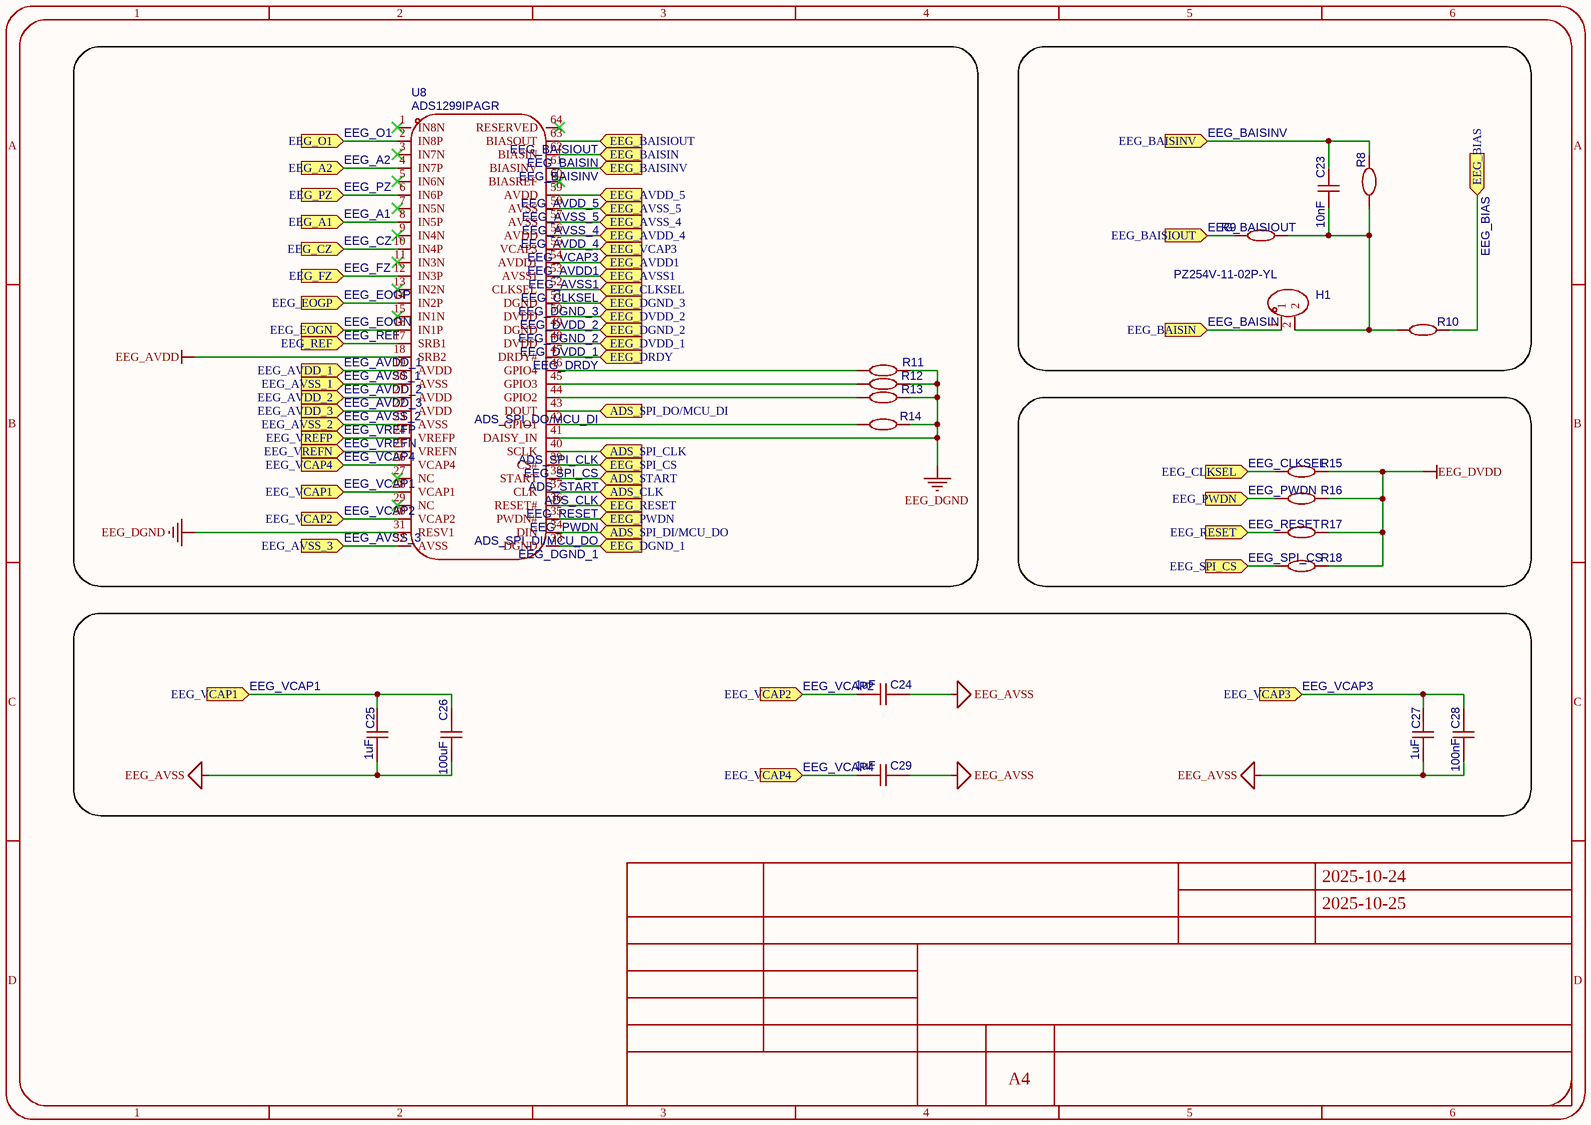
[diagram p0: MISC86293-4.schdoc]
# Altium project MISC86293-17.PrjPCB (part 2 of 3)

## Sheet MISC86293-4.schdoc
size 297 x 209 mm; @Create Time: 20:02:05; @Update Time: 00:34:01; @Board Name: MISC86293; Version: V1.0; @Project Name: MISC86293; @Page Count: 8; @Update Date: 2025-10-25; @Create Date: 2025-10-24; @Schematic Name: MISC86293; @Page No: 2

### Parts
C23  10nF  [C0402]
C24  1uF  [C0402]
C25  1uF  [C0402]
C26  100uF  [C1206]
C27  1uF  [C0402]
C28  100nF  [C0402]
C29  1uF  [C0402]
H1  PZ254V-11-02P-YL  [HDR-TH_2P-P2.54-V-M]
R8  (no value)  [R0402]
R9  (no value)  [R0402]
R10  (no value)  [R0402]
R11  (no value)  [R0402]
R12  (no value)  [R0402]
R13  (no value)  [R0402]
R14  (no value)  [R0402]
R15  (no value)  [R0402]
R16  (no value)  [R0402]
R17  (no value)  [R0402]
R18  (no value)  [R0402]
U8  ADS1299IPAGR  [TQFP-64_L10.0-W10.0-P0.50-LS12.0-TL]

### Ports
ADS_CLK (in), ADS_SPI_CLK (in), ADS_SPI_DI/MCU_DO (in), ADS_SPI_DO/MCU_DI (in), ADS_START (in), EEG_A1 (in), EEG_A2 (in), EEG_AVDD1 (in), EEG_AVDD_1 (in), EEG_AVDD_2 (in), EEG_AVDD_3 (in), EEG_AVDD_4 (in), EEG_AVDD_5 (in), EEG_AVSS1 (in), EEG_AVSS_1 (in), EEG_AVSS_2 (in), EEG_AVSS_3 (in), EEG_AVSS_4 (in), EEG_AVSS_5 (in), EEG_BAISIN (in), EEG_BAISINV (in), EEG_BAISIOUT (in), EEG_BIAS (in), EEG_CLKSEL (in), EEG_CZ (in), EEG_DGND_1 (in), EEG_DGND_2 (in), EEG_DGND_3 (in), EEG_DRDY (in), EEG_DVDD_1 (in), EEG_DVDD_2 (in), EEG_EOGN (in), EEG_EOGP (in), EEG_FZ (in), EEG_O1 (in), EEG_PWDN (in), EEG_PZ (in), EEG_REF (in), EEG_RESET (in), EEG_SPI_CS (in), EEG_VCAP1 (in), EEG_VCAP2 (in), EEG_VCAP3 (in), EEG_VCAP4 (in), EEG_VREFN (in), EEG_VREFP (in)

### Nets
EEG_AVDD1: U8.18(SRB2) U8.19(AVDD) U8.21(AVDD) U8.22(AVDD) U8.54(AVDD1) U8.56(AVDD) U8.59(AVDD) ; port EEG_AVDD_1, port EEG_AVDD_2, port EEG_AVDD_3, port EEG_AVDD_4, port EEG_AVDD_5, port EEG_AVDD1  [also labelled EEG_AVDD, EEG_AVDD_1, EEG_AVDD_2, EEG_AVDD_3, EEG_AVDD_4, EEG_AVDD_5]
EEG_AVSS1: C24.2 C25.1 C26.1 C27.1 C28.1 C29.2 U8.20(AVSS) U8.23(AVSS) U8.25(VREFN) U8.32(AVSS) U8.53(AVSS1) U8.57(AVSS) U8.58(AVSS) ; port EEG_AVSS_1, port EEG_AVSS_2, port EEG_AVSS_4, port EEG_AVSS_5, port EEG_AVSS1, port EEG_VREFN, port EEG_AVSS_3  [also labelled EEG_AVSS, EEG_AVSS_1, EEG_AVSS_2, EEG_AVSS_3, EEG_AVSS_4, EEG_AVSS_5, EEG_VREFN]
EEG_DGND_1: R11.2 R12.2 R13.2 R14.2 U8.31(RESV1) U8.33(DGND) U8.41(DAISY_IN) U8.49(DGND) U8.51(DGND) ; port EEG_DGND_1, port EEG_DGND_2, port EEG_DGND_3  [also labelled EEG_DGND, EEG_DGND_2, EEG_DGND_3]
EEG_DVDD_1: R15.2 R16.2 R17.2 R18.2 U8.48(DVDD) U8.50(DVDD) ; port EEG_DVDD_1, port EEG_DVDD_2  [also labelled EEG_DVDD, EEG_DVDD_2]
ADS_CLK: U8.37(CLK) ; port ADS_CLK
ADS_SPI_CLK: U8.40(SCLK) ; port ADS_SPI_CLK
ADS_SPI_DI/MCU_DO: U8.34(DIN) ; port ADS_SPI_DI/MCU_DO
ADS_SPI_DO/MCU_DI: U8.43(DOUT) ; port ADS_SPI_DO/MCU_DI
ADS_START: U8.38(START) ; port ADS_START
EEG_A1: U8.8(IN5P) ; port EEG_A1
EEG_A2: U8.4(IN7P) ; port EEG_A2
EEG_BAISIN: H1.1 U8.62(BIASIN) ; port EEG_BAISIN
EEG_BAISINV: C23.2 R8.1 U8.61(BIASINV) ; port EEG_BAISINV
EEG_BAISIOUT: R9.1 U8.63(BIASOUT) ; port EEG_BAISIOUT
EEG_BIAS: R10.2 ; port EEG_BIAS
EEG_CLKSEL: R15.1 U8.52(CLKSEL) ; port EEG_CLKSEL
EEG_CZ: U8.10(IN4P) ; port EEG_CZ
EEG_DRDY: U8.47(DRDY#) ; port EEG_DRDY
EEG_EOGN: U8.16(IN1P) ; port EEG_EOGN
EEG_EOGP: U8.14(IN2P) ; port EEG_EOGP
EEG_FZ: U8.12(IN3P) ; port EEG_FZ
EEG_O1: U8.2(IN8P) ; port EEG_O1
EEG_PWDN: R16.1 U8.35(PWDN#) ; port EEG_PWDN
EEG_PZ: U8.6(IN6P) ; port EEG_PZ
EEG_REF: U8.17(SRB1) ; port EEG_REF
EEG_RESET: R17.1 U8.36(RESET#) ; port EEG_RESET
EEG_SPI_CS: R18.1 U8.39(CS#) ; port EEG_SPI_CS
EEG_VCAP1: C25.2 C26.2 U8.28(VCAP1) ; port EEG_VCAP1
EEG_VCAP2: C24.1 U8.30(VCAP2) ; port EEG_VCAP2
EEG_VCAP3: C27.2 C28.2 U8.55(VCAP3) ; port EEG_VCAP3
EEG_VCAP4: C29.1 U8.26(VCAP4) ; port EEG_VCAP4
EEG_VREFP: U8.24(VREFP) ; port EEG_VREFP
NetC23_1: C23.1 H1.2 R8.2 R9.2 R10.1
NetR11_1: R11.1 U8.46(GPIO4)
NetR12_1: R12.1 U8.45(GPIO3)
NetR13_1: R13.1 U8.44(GPIO2)
NetR14_1: R14.1 U8.42(GPIO1)

Not connected (* = marked no-connect by the designer): U8 1(IN8N)* 3(IN7N)* 5(IN6N)* 7(IN5N)* 9(IN4N)* 11(IN3N)* 13(IN2N)* 15(IN1N)* 27(NC)* 29(NC)* 60(BIASREF)* 64(RESERVED)*

### Notes on the sheet
- 1
- 2
- 3
- 4
- 5
- 6
- A
- B
- C
- 2025-10-24
- 2025-10-25
- D
- A4

### Library data of the parts
C23 = CL05B103KB5NNNC: Symbol: CC0402KRX7R9BB152; AddInBom: yes; ModelId: 36a51122f27c49738f86b3bfa98863e0; ModelName: C0402_L1.0-W0.5-H0.5; ModelTransform: 39.37,19.685,0,0,0,0,0,0,0; Voltage Rating: 50V; Temperature Coefficient: X7R; Device: CL05B103KB5NNNC; Supplier: LCSC; Manufacturer Part: CL05B103KB5NNNC; Value: 10nF; Supplier Part: C15195; JLCPCB Part Class: Basic Part; Supplier Footprint: 0402; Datasheet: https://item.szlcsc.com/datasheet/CL05B103KB5NNNC/15869.html; ConvertToPcb: yes; FootprintName: C0402
C24 C25 C27 C29 = GRM155Z71A105KE01D: AddInBom: yes; ModelId: 36a51122f27c49738f86b3bfa98863e0; ModelName: C0402_L1.0-W0.5-H0.5; ModelTransform: 39.37,19.685,0,0,0,0,0,0,0; Voltage Rated: 10V; Temperature Coefficient: X7R; Symbol: GRM155Z71A105KE01D; Device: GRM155Z71A105KE01D; SupplierPart: C528974; ManufacturerPart: GRM155Z71A105KE01D; Supplier Footprint: 0402; Datasheet: https://atta.szlcsc.com/upload/public/pdf/source/20200508/C528974_15BC5D9F0CC13FAE313D74FE55DE6D9B.pdf; Supplier: LCSC; ConvertToPcb: yes; FootprintName: C0402; Value: 1uF
C26 = GRM31CR61A107ME05L: AddInBom: yes; ModelId: e4be705b945545a48e666415e3682bd8; ModelName: C1206_L3.2-W1.6-H1.3; ModelTransform: 125.984,62.992,0,0,0,0,0,0,0; Voltage Rated: 10V; Temperature Coefficient: X5R; Symbol: GRM31CR61A107ME05L; Device: GRM31CR61A107ME05L; Supplier: LCSC; Supplier Part: C312983; Manufacturer Part: GRM31CR61A107ME05L; Value: 100uF; Supplier Footprint: 1206; Datasheet: https://atta.szlcsc.com/upload/public/pdf/source/20181029/C312983_F99DFC7E8AF2C04CC95A01A8A93C8DA6.pdf; ConvertToPcb: yes; FootprintName: C1206
C28 = CL05B104KB54PNC: AddInBom: yes; ModelId: 36a51122f27c49738f86b3bfa98863e0; ModelName: C0402_L1.0-W0.5-H0.5; ModelTransform: 39.37,19.685,0,0,0,0,0,0,0; Voltage Rated: 50V; Temperature Coefficient: X7R; Device: CL05B104KB54PNC; Symbol: CL05B104KB54PNC; SupplierPart: C307331; ManufacturerPart: CL05B104KB54PNC; Supplier Footprint: 0402; Datasheet: https://atta.szlcsc.com/upload/public/pdf/source/20160218/1457707763339.pdf; Supplier: LCSC; ConvertToPcb: yes; FootprintName: C0402; Value: 100nF
H1 = PZ254V-11-02P-YL: AddInBom: yes; ModelId: e35305ec3aa84b66b849f914b715e73f; ModelName: HDR2.54-M-LI-1X2P; ModelTransform: 200,100,0,0,0,0,0,0,-118.11; Pin Structure: 1x2P; Pitch: 2.54mm; Current Rating: 3A; Symbol: PZ254V-11-02P-YL; Device: PZ254V-11-02P-YL; SupplierPart: C41425305; ManufacturerPart: PZ254V-11-02P-YL; Datasheet: https://item.szlcsc.com/datasheet/PZ254V-11-02P-YL/43268222.html; Supplier: LCSC; ConvertToPcb: yes; FootprintName: HDR-TH_2P-P2.54-V-M; Number of Pins: 2P; Length of Mating Pin: 6.1mm; Insulation Height: 2.5mm; Length of End Connection Pin: 3mm
R8 = FRC0402F3923TS: Symbol: SC0402F1004F2ANRH; AddInBom: yes; ModelId: 98c88bc2b9094f218f3a3e30a7012738; ModelName: R0402_L1.0-W0.5-H0.4; ModelTransform: 39.37,19.685,0,0,0,0,0,0,0; Power(Watts): 62.5mW; Voltage-Supply(Max): 50V; Device: FRC0402F3923TS; SupplierPart: C5713271; ManufacturerPart: FRC0402F3923TS; Supplier Footprint: 0402; JLCPCB Part Class: Extended Part; Supplier: LCSC; ConvertToPcb: yes; FootprintName: R0402
R9 = 0402WGF0000TCE: AddInBom: yes; ModelId: 671aefced39d4c318694bba8bd8efd39; ModelName: R0402_L1.0-W0.5-H0.5; ModelTransform: 39.37,19.685,0,0,0,0,0,0.0005,0; Power(Watts): 62.5mW; Overload Voltage (Max): 50V; Symbol: 0402WGF0000TCE; Device: 0402WGF0000TCE; Supplier: LCSC; Manufacturer Part: 0402WGF0000TCE; Supplier Part: C17168; Supplier Footprint: 0402; Datasheet: https://atta.szlcsc.com/upload/public/pdf/source/20200306/C422600_1E6D84923E4A46A82E41ADD87F860B5C.pdf; ConvertToPcb: yes; FootprintName: R0402
R10 = RC0402FR-07100KL: AddInBom: yes; ModelId: 671aefced39d4c318694bba8bd8efd39; ModelName: R0402_L1.0-W0.5-H0.5; ModelTransform: 39.37,19.685,0,0,0,0,0,0.0005,0; Power(Watts): 62.5mW; Overload Voltage (Max): 50V; Device: RC0402FR-07100KL; Symbol: RC0402FR-07100KL; SupplierPart: C60491; ManufacturerPart: RC0402FR-07100KL; Supplier Footprint: 0402; JLCPCB Part Class: Extended Part; Datasheet: https://atta.szlcsc.com/upload/public/pdf/source/20180927/C295883_E8D83085EA81BD7DE0B2B681138C15EE.pdf; Supplier: LCSC; ConvertToPcb: yes; FootprintName: R0402
R11-R18 = RC0402FR-0710KL: AddInBom: yes; ModelId: 671aefced39d4c318694bba8bd8efd39; ModelName: R0402_L1.0-W0.5-H0.5; ModelTransform: 39.37,19.685,0,0,0,0,0,0.0005,0; Power(Watts): 62.5mW; Overload Voltage (Max): 50V; Symbol: RC0402FR-0710KL; Device: RC0402FR-0710KL; SupplierPart: C60490; ManufacturerPart: RC0402FR-0710KL; Supplier Footprint: 0402; Datasheet: https://atta.szlcsc.com/upload/public/pdf/source/20170925/C131467_1506321478108990263.pdf; Supplier: LCSC; ConvertToPcb: yes; FootprintName: R0402
U8 = ADS1299IPAGR: Symbol: ADS1299-6PAG; AddInBom: yes; ModelId: 8d2ba6bfb2a14fb7921a74871619a185; ModelName: TQFP-64_L10.0-W10.0-H1.2-LS12.0-P0.50; ModelTransform: 473.00941,473.00941,0,0,0,0,0.039,0,0; Voltage - Supply: 4.75V~5.25V; S/N Ratio: 121dB; Device: ADS1299IPAGR; SupplierPart: C476817; ManufacturerPart: ADS1299IPAGR; Supplier Footprint: TQFP-64(10x10); JLCPCB Part Class: Extended Part; Datasheet: https://www.ti.com/cn/lit/gpn/ads1299; Supplier: LCSC; ConvertToPcb: yes; FootprintName: TQFP-64_L10.0-W10.0-P0.50-LS12.0-TL

## Sheet MISC86293-12.schdoc
size 297 x 209 mm; @Create Time: 20:02:05; @Update Time: 00:34:01; @Board Name: MISC86293; Version: V1.0; @Project Name: MISC86293; @Page Count: 8; @Update Date: 2025-10-25; @Create Date: 2025-10-24; @Schematic Name: MISC86293; @Page No: 7
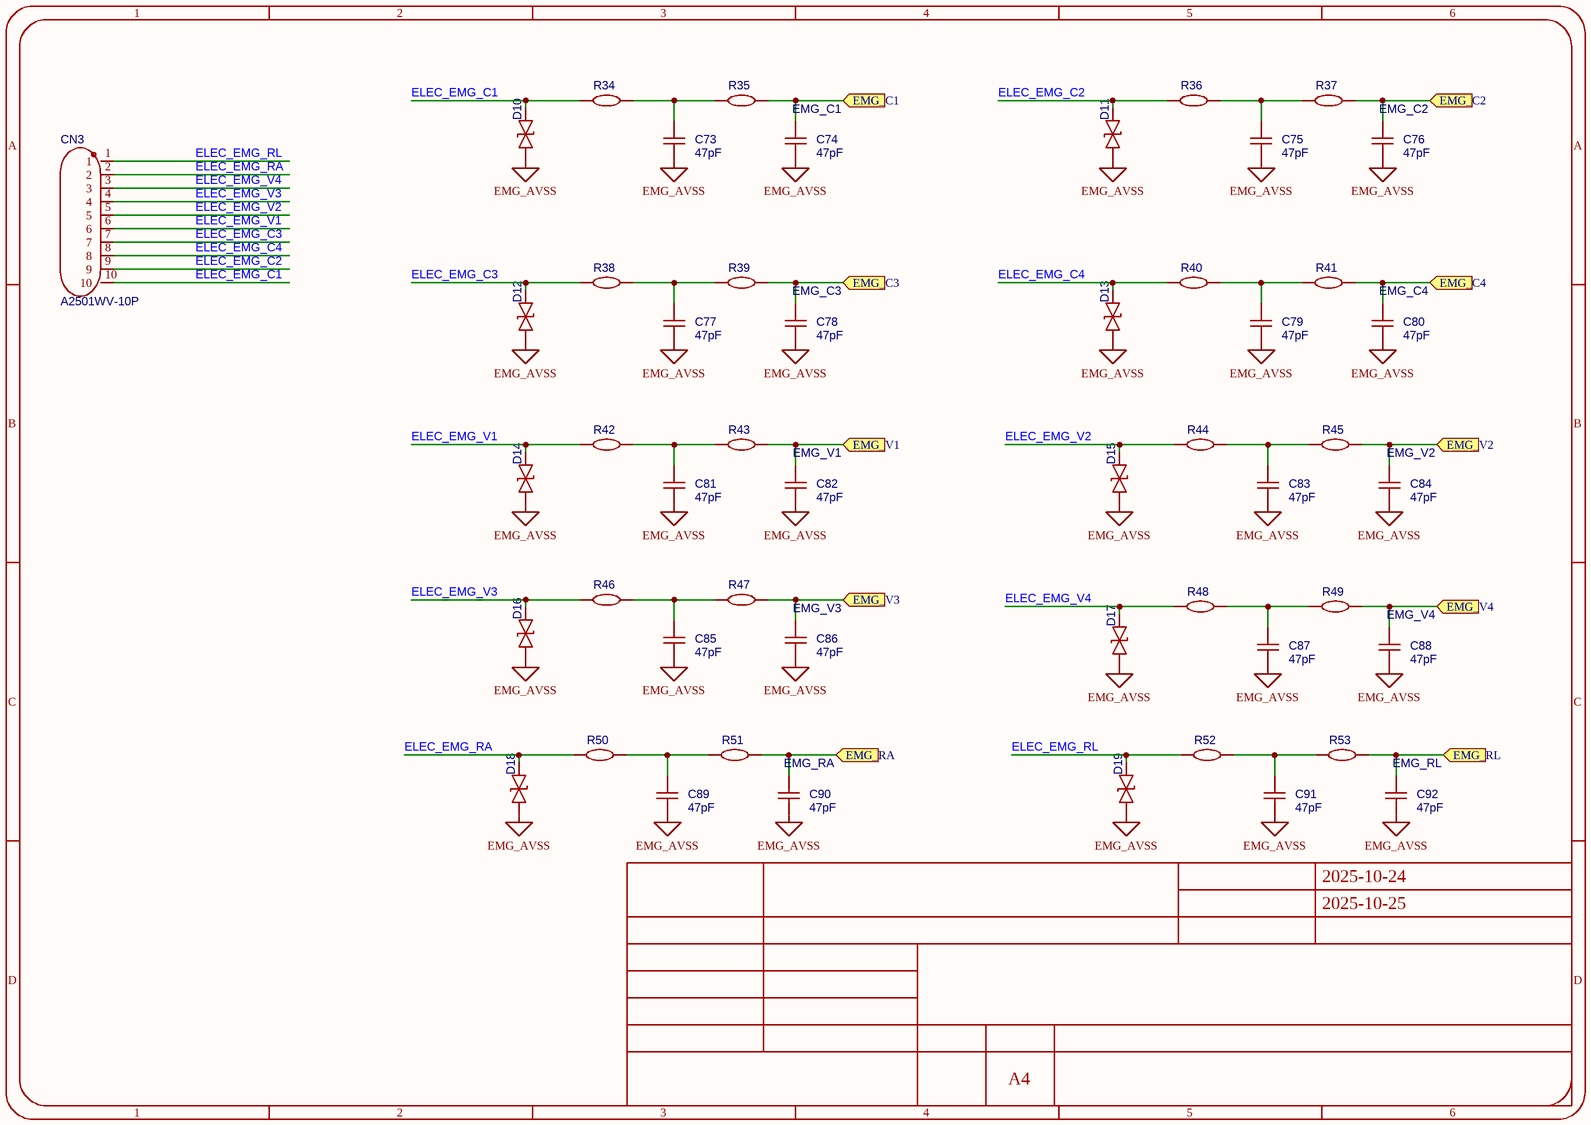
[diagram p1: MISC86293-12.schdoc]

### Parts
C73  47pF  [C0402]
C74  47pF  [C0402]
C75  47pF  [C0402]
C76  47pF  [C0402]
C77  47pF  [C0402]
C78  47pF  [C0402]
C79  47pF  [C0402]
C80  47pF  [C0402]
C81  47pF  [C0402]
C82  47pF  [C0402]
C83  47pF  [C0402]
C84  47pF  [C0402]
C85  47pF  [C0402]
C86  47pF  [C0402]
C87  47pF  [C0402]
C88  47pF  [C0402]
C89  47pF  [C0402]
C90  47pF  [C0402]
C91  47pF  [C0402]
C92  47pF  [C0402]
CN3  A2501WV-10P  [CONN-TH_A2501WV-10P]
D10  TPD1E10B06DPYR-TP  [X1-DFN1006-2_L1.0-W0.6-BI]  (value not drawn)
D11  TPD1E10B06DPYR-TP  [X1-DFN1006-2_L1.0-W0.6-BI]  (value not drawn)
D12  TPD1E10B06DPYR-TP  [X1-DFN1006-2_L1.0-W0.6-BI]  (value not drawn)
D13  TPD1E10B06DPYR-TP  [X1-DFN1006-2_L1.0-W0.6-BI]  (value not drawn)
D14  TPD1E10B06DPYR-TP  [X1-DFN1006-2_L1.0-W0.6-BI]  (value not drawn)
D15  TPD1E10B06DPYR-TP  [X1-DFN1006-2_L1.0-W0.6-BI]  (value not drawn)
D16  TPD1E10B06DPYR-TP  [X1-DFN1006-2_L1.0-W0.6-BI]  (value not drawn)
D17  TPD1E10B06DPYR-TP  [X1-DFN1006-2_L1.0-W0.6-BI]  (value not drawn)
D18  TPD1E10B06DPYR-TP  [X1-DFN1006-2_L1.0-W0.6-BI]  (value not drawn)
D19  TPD1E10B06DPYR-TP  [X1-DFN1006-2_L1.0-W0.6-BI]  (value not drawn)
R34  (no value)  [R0402]
R35  (no value)  [R0402]
R36  (no value)  [R0402]
R37  (no value)  [R0402]
R38  (no value)  [R0402]
R39  (no value)  [R0402]
R40  (no value)  [R0402]
R41  (no value)  [R0402]
R42  (no value)  [R0402]
R43  (no value)  [R0402]
R44  (no value)  [R0402]
R45  (no value)  [R0402]
R46  (no value)  [R0402]
R47  (no value)  [R0402]
R48  (no value)  [R0402]
R49  (no value)  [R0402]
R50  (no value)  [R0402]
R51  (no value)  [R0402]
R52  (no value)  [R0402]
R53  (no value)  [R0402]

### Ports
EMG_C1 (in), EMG_C2 (in), EMG_C3 (in), EMG_C4 (in), EMG_RA (in), EMG_RL (in), EMG_V1 (in), EMG_V2 (in), EMG_V3 (in), EMG_V4 (in)

### Nets
EMG_AVSS: C73.1 C74.1 C75.1 C76.1 C77.1 C78.1 C79.1 C80.1 C81.1 C82.1 C83.1 C84.1 C85.1 C86.1 C87.1 C88.1 C89.1 C90.1 C91.1 C92.1 D10.1 D11.1 D12.1 D13.1 D14.1 D15.1 D16.1 D17.1 D18.1 D19.1  [project net EMG_AVSS1]
ELEC_EMG_C1: CN3.10 D10.2 R34.1
ELEC_EMG_C2: CN3.9 D11.2 R36.1
ELEC_EMG_C3: CN3.7 D12.2 R38.1
ELEC_EMG_C4: CN3.8 D13.2 R40.1
ELEC_EMG_RA: CN3.2 D18.2 R50.1
ELEC_EMG_RL: CN3.1 D19.2 R52.1
ELEC_EMG_V1: CN3.6 D14.2 R42.1
ELEC_EMG_V2: CN3.5 D15.2 R44.1
ELEC_EMG_V3: CN3.4 D16.2 R46.1
ELEC_EMG_V4: CN3.3 D17.2 R48.1
EMG_C1: C74.2 R35.2 ; port EMG_C1
EMG_C2: C76.2 R37.2 ; port EMG_C2
EMG_C3: C78.2 R39.2 ; port EMG_C3
EMG_C4: C80.2 R41.2 ; port EMG_C4
EMG_RA: C90.2 R51.2 ; port EMG_RA
EMG_RL: C92.2 R53.2 ; port EMG_RL
EMG_V1: C82.2 R43.2 ; port EMG_V1
EMG_V2: C84.2 R45.2 ; port EMG_V2
EMG_V3: C86.2 R47.2 ; port EMG_V3
EMG_V4: C88.2 R49.2 ; port EMG_V4
NetC73_2: C73.2 R34.2 R35.1
NetC75_2: C75.2 R36.2 R37.1
NetC77_2: C77.2 R38.2 R39.1
NetC79_2: C79.2 R40.2 R41.1
NetC81_2: C81.2 R42.2 R43.1
NetC83_2: C83.2 R44.2 R45.1
NetC85_2: C85.2 R46.2 R47.1
NetC87_2: C87.2 R48.2 R49.1
NetC89_2: C89.2 R50.2 R51.1
NetC91_2: C91.2 R52.2 R53.1

### Notes on the sheet
- 1
- 2
- 3
- 4
- 5
- 6
- A
- B
- C
- 2025-10-24
- 2025-10-25
- D
- A4

### Library data of the parts
C73-C92 = 0402CG470J500NT: AddInBom: yes; ModelId: 36a51122f27c49738f86b3bfa98863e0; ModelName: C0402_L1.0-W0.5-H0.5; ModelTransform: 39.37,19.685,0,0,0,0,0,0,0; Voltage Rating: 50V; Temperature Coefficient: C0G; Symbol: 0402CG470J500NT; Device: 0402CG470J500NT; SupplierPart: C1567; ManufacturerPart: 0402CG470J500NT; Supplier Footprint: 0402; Datasheet: https://item.szlcsc.com/datasheet/0402CG470J500NT/1919.html; Supplier: LCSC; ConvertToPcb: yes; FootprintName: C0402; Value: 47pF
CN3 = A2501WV-10P: AddInBom: yes; ModelId: 8fed046ffe3f4aaeaaccc95f13076c79; ModelTransform: 1082.675,224.409,0,0,0,0,0,22.205,-137.795; Pins Structure: 1x10P; Pitch: 2.5mm; Reference Series: XH; Number of PINs Per Row: 10; Current Rating: 3A; Voltage Rating: 250V; Plastic Material: PA66; Flame Retardant Rating: UL94V-0; Symbol: A2501WV-10P; Device: A2501WV-10P; SupplierPart: C225396; ManufacturerPart: A2501WV-10P; Datasheet: https://item.szlcsc.com/datasheet/A2501WV-10P/225679.html; Supplier: LCSC; ConvertToPcb: yes; FootprintName: CONN-TH_A2501WV-10P; ModelName: CONN-TH_A2501WV-10P; Number of Pins: 10P; Number of Rows: 1; Row Spacing: -; Color: -
D10-D19 = TPD1E10B06DPYR-TP: AddInBom: yes; ModelId: be5a8b78c3cb4e51be1cd7cc83308da0; ModelName: X1-DFN1006-2_L1.0-W0.6-H0.5-BI; ModelTransform: 40.1574,24.4094,0,0,0,0,0,0,0; Symbol: TPD1E10B06DPYR-TP; Device: TPD1E10B06DPYR-TP; Supplier: LCSC; Supplier Part: C558445; Manufacturer Part: TPD1E10B06DPYR-TP; LCSC Part Name: TPD1E10B06DPYR-TP; Supplier Footprint: X1-DFN1006-2; Datasheet: https://atta.szlcsc.com/upload/public/pdf/source/20230621/7FCA3FDEAE9F1BA71F34C850D9682567.pdf; ConvertToPcb: yes; FootprintName: X1-DFN1006-2_L1.0-W0.6-BI
R34 R36 R38 R40 R42 R44 R46 R48 R50 R52 = AC0402FR-0722K1L: AddInBom: yes; ModelId: 98c88bc2b9094f218f3a3e30a7012738; ModelName: R0402_L1.0-W0.5-H0.4; ModelTransform: 39.37,19.685,0,0,0,0,0,0,0; Power(Watts): 62.5mW; Voltage-Supply(Max): 50V; Symbol: AC0402FR-0722K1L; Device: AC0402FR-0722K1L; SupplierPart: C226356; ManufacturerPart: AC0402FR-0722K1L; Supplier Footprint: 0402; Datasheet: https://item.szlcsc.com/datasheet/AC0402FR-0722K1L/227126.html; Supplier: LCSC; ConvertToPcb: yes; FootprintName: R0402
R35 R37 R39 R41 R43 R45 R47 R49 R51 R53 = 0402WGF1002TCE: AddInBom: yes; ModelId: 98c88bc2b9094f218f3a3e30a7012738; ModelName: R0402_L1.0-W0.5-H0.4; ModelTransform: 39.37,19.685,0,0,0,0,0,0,0; Power(Watts): 62.5mW; Voltage-Supply(Max): 50V; Symbol: 0402WGF1002TCE; Device: 0402WGF1002TCE; SupplierPart: C25744; ManufacturerPart: 0402WGF1002TCE; Supplier Footprint: 0402; Datasheet: https://item.szlcsc.com/datasheet/0402WGF1002TCE/26487.html; Supplier: LCSC; ConvertToPcb: yes; FootprintName: R0402

## Sheet MISC86293-21.schdoc
size 297 x 209 mm; Version: V1.0; @Project Name: MISC86293; @Page Count: 8; @Update Date: 2025-10-25; @Create Date: 2025-10-24; @Schematic Name: MISC86293; @Page No: 8; @Create Time: 20:02:06; @Update Time: 00:34:01; @Board Name: MISC86293
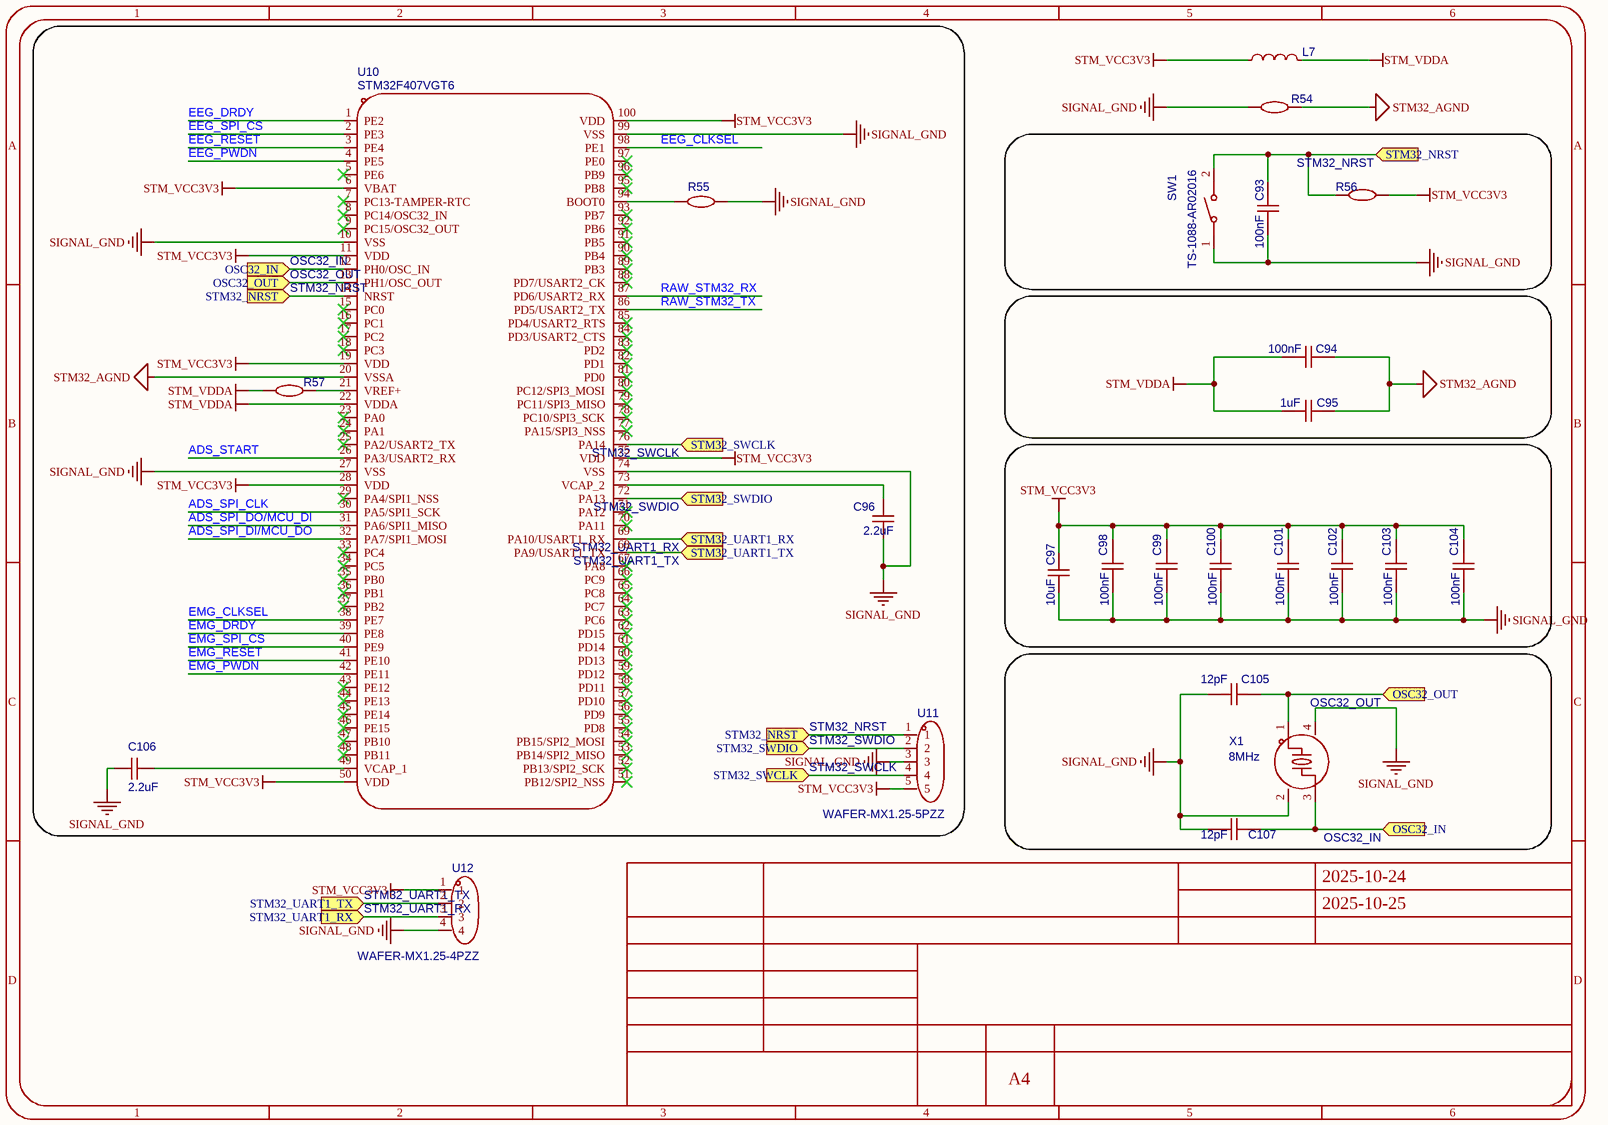
[diagram p2: MISC86293-21.schdoc]

### Parts
C93  100nF  [C0402]
C94  100nF  [C0402]
C95  1uF  [C0402]
C96  2.2uF  [C0603]
C97  10uF  [C0603]
C98  100nF  [C0402]
C99  100nF  [C0402]
C100  100nF  [C0402]
C101  100nF  [C0402]
C102  100nF  [C0402]
C103  100nF  [C0402]
C104  100nF  [C0402]
C105  12pF  [C0402]
C106  2.2uF  [C0603]
C107  12pF  [C0402]
L7  GZ1608D601TF  [L0603]  (value not drawn)
R54  (no value)  [R0402]
R55  (no value)  [R0402]
R56  (no value)  [R0402]
R57  (no value)  [R0402]
SW1  TS-1088-AR02016  [SW-SMD_L3.9-W3.0-P4.45]
U10  STM32F407VGT6  [LQFP-100_L14.0-W14.0-P0.50-LS16.0-BL]
U11  WAFER-MX1.25-5PZZ  [CONN-TH_5P-P1.25_XUNPU_WAFER-MX1.25-5PZZ]
U12  WAFER-MX1.25-4PZZ  [CONN-TH_4P-P1.25_WAFER-MX1.25-4PZZ]
X1  8MHz  [CRYSTAL-SMD_4P-L3.2-W2.5-BL]

### Ports
OSC32_IN (in), OSC32_OUT (in), STM32_NRST (in), STM32_SWCLK (in), STM32_SWDIO (in), STM32_UART1_RX (in), STM32_UART1_TX (in)

### Nets
SIGNAL_GND: C93.1 C96.1 C97.1 C98.1 C99.1 C100.1 C101.1 C102.1 C103.1 C104.1 C105.1 C106.2 C107.1 R54.1 R55.2 SW1.1 U10.10(VSS) U10.27(VSS) U10.74(VSS) U10.99(VSS) U11.3 U12.4 X1.2(GND) X1.4(GND)
STM32_AGND: C94.1 C95.1 R54.2 U10.20(VSSA)
STM_VCC3V3: C97.2 C98.2 C99.2 C100.2 C101.2 C102.2 C103.2 C104.2 L7.1 R56.2 U10.6(VBAT) U10.11(VDD) U10.19(VDD) U10.28(VDD) U10.50(VDD) U10.75(VDD) U10.100(VDD) U11.5 U12.1
STM_VDDA: C94.2 C95.2 L7.2 R57.1 U10.22(VDDA)
ADS_SPI_CLK: U10.30(PA5/SPI1_SCK)
ADS_SPI_DI/MCU_DO: U10.32(PA7/SPI1_MOSI)
ADS_SPI_DO/MCU_DI: U10.31(PA6/SPI1_MISO)
ADS_START: U10.26(PA3/USART2_RX)
EEG_CLKSEL: U10.98(PE1)
EEG_DRDY: U10.1(PE2)
EEG_PWDN: U10.4(PE5)
EEG_RESET: U10.3(PE4)
EEG_SPI_CS: U10.2(PE3)
EMG_CLKSEL: U10.38(PE7)
EMG_DRDY: U10.39(PE8)
EMG_PWDN: U10.42(PE11)
EMG_RESET: U10.41(PE10)
EMG_SPI_CS: U10.40(PE9)
OSC32_IN: C107.2 U10.12(PH0/OSC_IN) X1.3 ; port OSC32_IN
OSC32_OUT: C105.2 U10.13(PH1/OSC_OUT) X1.1 ; port OSC32_OUT
RAW_STM32_RX: U10.87(PD6/USART2_RX)
RAW_STM32_TX: U10.86(PD5/USART2_TX)
STM32_NRST: C93.2 R56.1 SW1.2 U10.14(NRST) U11.1 ; port STM32_NRST
STM32_SWCLK: U10.76(PA14) U11.4 ; port STM32_SWCLK
STM32_SWDIO: U10.72(PA13) U11.2 ; port STM32_SWDIO
STM32_UART1_RX: U10.69(PA10/USART1_RX) U12.3 ; port STM32_UART1_RX
STM32_UART1_TX: U10.68(PA9/USART1_TX) U12.2 ; port STM32_UART1_TX
NetC96_2: C96.2 U10.73(VCAP_2)
NetC106_1: C106.1 U10.49(VCAP_1)
NetR55_1: R55.1 U10.94(BOOT0)
NetR57_2: R57.2 U10.21(VREF+)

Not connected (* = marked no-connect by the designer): U10 5(PE6)* 7(PC13-TAMPER-RTC)* 8(PC14/OSC32_IN)* 9(PC15/OSC32_OUT)* 15(PC0)* 16(PC1)* 17(PC2)* 18(PC3)* 23(PA0)* 24(PA1)* 25(PA2/USART2_TX)* 29(PA4/SPI1_NSS)* 33(PC4)* 34(PC5)* 35(PB0)* 36(PB1)* 37(PB2)* 43(PE12)* 44(PE13)* 45(PE14)* 46(PE15)* 47(PB10)* 48(PB11)* 51(PB12/SPI2_NSS)* 52(PB13/SPI2_SCK)* 53(PB14/SPI2_MISO)* 54(PB15/SPI2_MOSI)* 55(PD8)* 56(PD9)* 57(PD10)* 58(PD11)* 59(PD12)* 60(PD13)* 61(PD14)* 62(PD15)* 63(PC6)* 64(PC7)* 65(PC8)* 66(PC9)* 67(PA8)* 70(PA11)* 71(PA12)* 77(PA15/SPI3_NSS)* 78(PC10/SPI3_SCK)* 79(PC11/SPI3_MISO)* 80(PC12/SPI3_MOSI)* 81(PD0)* 82(PD1)* 83(PD2)* 84(PD3/USART2_CTS)* 85(PD4/USART2_RTS)* 88(PD7/USART2_CK)* 89(PB3)* 90(PB4)* 91(PB5)* 92(PB6)* 93(PB7)* 95(PB8)* 96(PB9)* 97(PE0)*

### Notes on the sheet
- 1
- 2
- 3
- 4
- 5
- 6
- A
- B
- C
- 2025-10-24
- 2025-10-25
- D
- A4

### Library data of the parts
C93 C94 C98-C104 = CC0402KRX7R7BB104: AddInBom: yes; ModelId: 36a51122f27c49738f86b3bfa98863e0; ModelName: C0402_L1.0-W0.5-H0.5; ModelTransform: 39.37,19.685,0,0,0,0,0,0,0; Voltage Rated: 16V; Temperature Coefficient: X7R; Symbol: CC0402KRX7R7BB104; Device: CC0402KRX7R7BB104; Supplier: LCSC; Manufacturer Part: CC0402KRX7R7BB104; Value: 100nF; Supplier Part: C60474; Supplier Footprint: 0402; Datasheet: https://atta.szlcsc.com/upload/public/pdf/source/20211223/9278FD768280B81DDBEF48FA36411A03.pdf; ConvertToPcb: yes; FootprintName: C0402
C95 = CC0402KRX5R6BB105: AddInBom: yes; ModelId: 36a51122f27c49738f86b3bfa98863e0; ModelName: C0402_L1.0-W0.5-H0.5; ModelTransform: 39.37,19.685,0,0,0,0,0,0,0; Voltage Rated: 10V; Temperature Coefficient: X5R; Symbol: CC0402KRX5R6BB105; Device: CC0402KRX5R6BB105; SupplierPart: C106254; ManufacturerPart: CC0402KRX5R6BB105; Supplier Footprint: 0402; Datasheet: https://atta.szlcsc.com/upload/public/pdf/source/20170914/C128857_1505359892143968080.pdf; Supplier: LCSC; ConvertToPcb: yes; FootprintName: C0402; Value: 1uF
C96 C106 = 0603B225K160NT: AddInBom: yes; ModelId: ac125912035d415993ca9572d50418b1; ModelName: C0603_L1.6-W0.8-H0.8; ModelTransform: 62.992,31.496,0,0,0,0,0,0,0; Voltage Rated: 16V; Temperature Coefficient: X7R; Symbol: 0603B225K160NT; Device: 0603B225K160NT; SupplierPart: C43922; ManufacturerPart: 0603B225K160NT; Supplier Footprint: 0603; Datasheet: https://atta.szlcsc.com/upload/public/pdf/source/20200305/C486355_26A10D38EF8C2A5C37091D0039909270.pdf; Supplier: LCSC; ConvertToPcb: yes; FootprintName: C0603; Value: 2.2uF
C97 = 0603X106K100NT: AddInBom: yes; ModelId: ac125912035d415993ca9572d50418b1; ModelName: C0603_L1.6-W0.8-H0.8; ModelTransform: 62.992,31.496,0,0,0,0,0,0,0; Voltage Rated: 10V; Temperature Coefficient: X5R; Symbol: 0603X106K100NT; Device: 0603X106K100NT; SupplierPart: C38898; ManufacturerPart: 0603X106K100NT; Supplier Footprint: 0603; Datasheet: https://atta.szlcsc.com/upload/public/pdf/source/20200305/C486355_26A10D38EF8C2A5C37091D0039909270.pdf; Supplier: LCSC; ConvertToPcb: yes; FootprintName: C0603; Value: 10uF
C105 C107 = AC0402JRNPO9BN120: AddInBom: yes; ModelId: 36a51122f27c49738f86b3bfa98863e0; ModelName: C0402_L1.0-W0.5-H0.5; ModelTransform: 39.37,19.685,0,0,0,0,0,0,0; Voltage Rated: 50V; Temperature Coefficient: NP0; Symbol: AC0402JRNPO9BN120; Device: AC0402JRNPO9BN120; SupplierPart: C726119; ManufacturerPart: AC0402JRNPO9BN120; Supplier Footprint: 0402; Datasheet: https://atta.szlcsc.com/upload/public/pdf/source/20200820/C726119_8498697DB4FD15A974AA7859FFEE439D.pdf; Supplier: LCSC; ConvertToPcb: yes; FootprintName: C0402; Value: 12pF
L7 = GZ1608D601TF: AddInBom: yes; ModelId: 2bc5ec593d464d6ba9807aec0b5673c2; ModelName: L0603_L1.6-W0.8-H0.5_BEAD; ModelTransform: 62.992,31.496,0,180,0,0,0.094,0.629,0; Current Rating: 200mA; Circuits: 1; Symbol: GZ1608D601TF; Device: GZ1608D601TF; Supplier: LCSC; Manufacturer Part: GZ1608D601TF; Supplier Part: C1002; Supplier Footprint: 0603; Datasheet: https://atta.szlcsc.com/upload/public/pdf/source/20231030/9B6A3E87682CEC1FF6638DFAA81D73FA.pdf; ConvertToPcb: yes; FootprintName: L0603
R54 = 0402WGF0000TCE: as R9 on sheet MISC86293-4; Symbol: 0402WGF0000TCE; Device: 0402WGF0000TCE; Supplier: LCSC; Manufacturer Part: 0402WGF0000TCE; Supplier Part: C17168; Supplier Footprint: 0402; Datasheet: https://atta.szlcsc.com/upload/public/pdf/source/20200306/C422600_1E6D84923E4A46A82E41ADD87F860B5C.pdf; ConvertToPcb: yes; FootprintName: R0402
R55 R56 = RC0402FR-0710KL: as R11-R18 on sheet MISC86293-4; Symbol: RC0402FR-0710KL; Device: RC0402FR-0710KL; SupplierPart: C60490; ManufacturerPart: RC0402FR-0710KL; Supplier Footprint: 0402; Datasheet: https://atta.szlcsc.com/upload/public/pdf/source/20170925/C131467_1506321478108990263.pdf; Supplier: LCSC; ConvertToPcb: yes; FootprintName: R0402
R57 = 0402WGF470JTCE: AddInBom: yes; ModelId: 671aefced39d4c318694bba8bd8efd39; ModelName: R0402_L1.0-W0.5-H0.5; ModelTransform: 39.37,19.685,0,0,0,0,0,0.0005,0; Power(Watts): 62.5mW; Overload Voltage (Max): 50V; Symbol: 0402WGF470JTCE; Device: 0402WGF470JTCE; SupplierPart: C25118; ManufacturerPart: 0402WGF470JTCE; Supplier Footprint: 0402; Datasheet: https://atta.szlcsc.com/upload/public/pdf/source/20200306/C422600_1E6D84923E4A46A82E41ADD87F860B5C.pdf; Supplier: LCSC; ConvertToPcb: yes; FootprintName: R0402
SW1 = TS-1088-AR02016: AddInBom: yes; ModelId: b26698b69f274ffabef8a26c7d0e5dd1; ModelName: SW-SMD_L3.9-W2.9-H2.0-LS4.8; ModelTransform: 188.976,114.174,0,0,0,0,0,0,0; Operating Force: 160gf; Switch Length: 4mm; Switch Width: 3mm; Switch Height: 2mm; Contact Current: 50mA; Voltage Rating (DC): 12V; Symbol: TS-1088-AR02016; Device: TS-1088-AR02016; SupplierPart: C720477; ManufacturerPart: TS-1088-AR02016; Supplier Footprint: SMD; Datasheet: https://atta.szlcsc.com/upload/public/pdf/source/20200810/C720475_60D09DD6C54279ADDB2DC25100F1CC11.pdf; Supplier: LCSC; ConvertToPcb: yes; FootprintName: SW-SMD_L3.9-W3.0-P4.45
U10 = STM32F407VGT6: AddInBom: yes; ModelId: 469e6cc70557486dbd01fd12ff814964; ModelName: LQFP-100_L14.0-W14.0-H1.4-LS16.0-P0.50; ModelTransform: 629.92,629.92,0,0,0,0,0,0,0; CPU Core: CM4; Program Storage Size: 1MB; RAM Size: 192KB; GPIO Ports Number: 82; Operating Voltage Range: 1.8V~3.6V; CPU Maximum Speed: 168MHz; Program Memory Type: FLASH; ADC (Bit): 12bit; Device: STM32F407VGT6; LCSC Part Name: STM32F407VGT6; SupplierPart: C12345; ManufacturerPart: STM32F407VGT6; Supplier Footprint: LQFP-100(14x14); Datasheet: https://atta.szlcsc.com/upload/public/pdf/source/20201130/C919362_39400D478C258148B3DF984CE4A4041A.pdf; Supplier: LCSC; ConvertToPcb: yes; SymbolName: STM32F407VGT6; FootprintName: LQFP-100_L14.0-W14.0-P0.50-LS16.0-BL; DAC (Bit): 12bit; PWM (Bit): -; Internal Comparator: -; communication protocol: -; Real-Time Clock: -; CCP Capture/Compare: -; Secure Digital Input and Output: -
U11 = WAFER-MX1.25-5PZZ: AddInBom: yes; ModelId: c63db3478aed4752a741debd80040a41; ModelTransform: 320.8655,130.315,0,0,0,0,0,-15.748,-90.551; Pins Structure: 1x5P; Pitch: 1.25mm; Reference Series: PicoBlade(MX 1.25); Number of PINs Per Row: 5; Current Rating: 1A; Voltage Rating: 125V; Plastic Material: LCP; Flame Retardant Rating: UL94V-0; Z-Height of the Board: 4.6mm; X-Length of Bottom Edge on Board (Spacing Line): 8.15mm; Y-Width of Bottom Edge on Board: 3.3mm; Symbol: WAFER-MX1.25-5PZZ; Device: WAFER-MX1.25-5PZZ; SupplierPart: C3029398; ManufacturerPart: WAFER-MX1.25-5PZZ; Datasheet: https://item.szlcsc.com/datasheet/WAFER-MX1.25-5PZZ/3561410.html; Supplier: LCSC; ConvertToPcb: yes; FootprintName: CONN-TH_5P-P1.25_XUNPU_WAFER-MX1.25-5PZZ; ModelName: CONN-TH_5P-P1.25_XUNPU_WAFER-MX1.25-5PZZ; Number of Pins: 5P; Number of Rows: 1; Row Spacing: -; Supplementary Features: -
U12 = WAFER-MX1.25-4PZZ: AddInBom: yes; ModelId: e263fd5d797b4db8bb8c543a0fc3d47f; ModelTransform: 272.0467,129.921,0,0,0,0,-0.004,-15.982,-94.488; Pins Structure: 1x4P; Pitch: 1.25mm; Reference Series: PicoBlade(MX 1.25); Number of PINs Per Row: 4; Current Rating: 1A; Voltage Rating: 125V; Plastic Material: LCP; Flame Retardant Rating: UL94V-0; Z-Height of the Board: 4.6mm; X-Length of Bottom Edge on Board (Spacing Line): 6.9mm; Y-Width of Bottom Edge on Board: 3.3mm; Symbol: WAFER-MX1.25-4PZZ; Device: WAFER-MX1.25-4PZZ; SupplierPart: C3029397; ManufacturerPart: WAFER-MX1.25-4PZZ; Datasheet: https://item.szlcsc.com/datasheet/WAFER-MX1.25-4PZZ/3561409.html; Supplier: LCSC; ConvertToPcb: yes; FootprintName: CONN-TH_4P-P1.25_WAFER-MX1.25-4PZZ; ModelName: CONN-TH_4P-P1.25_WAFER-MX1.25-4PZZ; Number of Pins: 4P; Number of Rows: 1; Row Spacing: -; Supplementary Features: -
X1 = X32258MOB4SI: AddInBom: yes; ModelId: 02485e56ba8d4732a26526d2983fc729; ModelTransform: 125.984,98.425,0,0,0,0,0,0,0; Load Capacitance: 12pF; Symbol: X32258MOB4SI; Device: X32258MOB4SI; SupplierPart: C2682775; ManufacturerPart: X32258MOB4SI; Supplier Footprint: SMD3225-4P; JLCPCB Part Class: Extended Part; Datasheet: https://item.szlcsc.com/datasheet/X32258MOB4SI/2777872.html; Supplier: LCSC; ConvertToPcb: yes; FootprintName: CRYSTAL-SMD_4P-L3.2-W2.5-BL; ModelName: CRYSTAL-SMD_4P-L3.2-W2.5-BL; Value: 8MHz